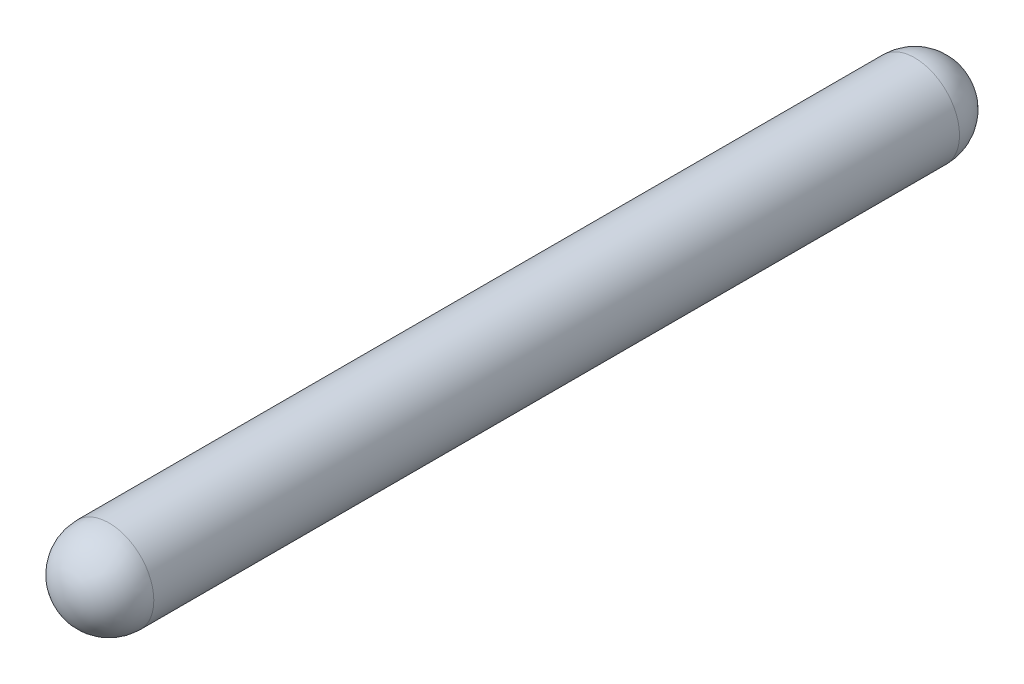
SolidWorks part; units mm, degrees
ref_plane "Front Plane" through (0, 0, 0) normal (0, 0, 1) x (1, 0, 0)
ref_plane "Top Plane" through (0, 0, 0) normal (0, 1, 0) x (1, 0, 0)
ref_plane "Right Plane" through (0, 0, 0) normal (1, 0, 0) x (0, 0, -1)
sketch "Sketch1" plane through (0, 0, 0) normal (0, 0, 1) x (1, 0, 0)
  circle A1 centre (-91.3, 42) radius 1 construction
  circle A2 centre (-91.3, 42) radius 1
extrude "Boss-Extrude1" add sketch "Sketch1" against normal mid plane 20 from offset 15 offset against normal yes
fillet "Fillet1" radius 1 2 edges at (-90.3, 42, -25) (-90.3, 42, -5)
